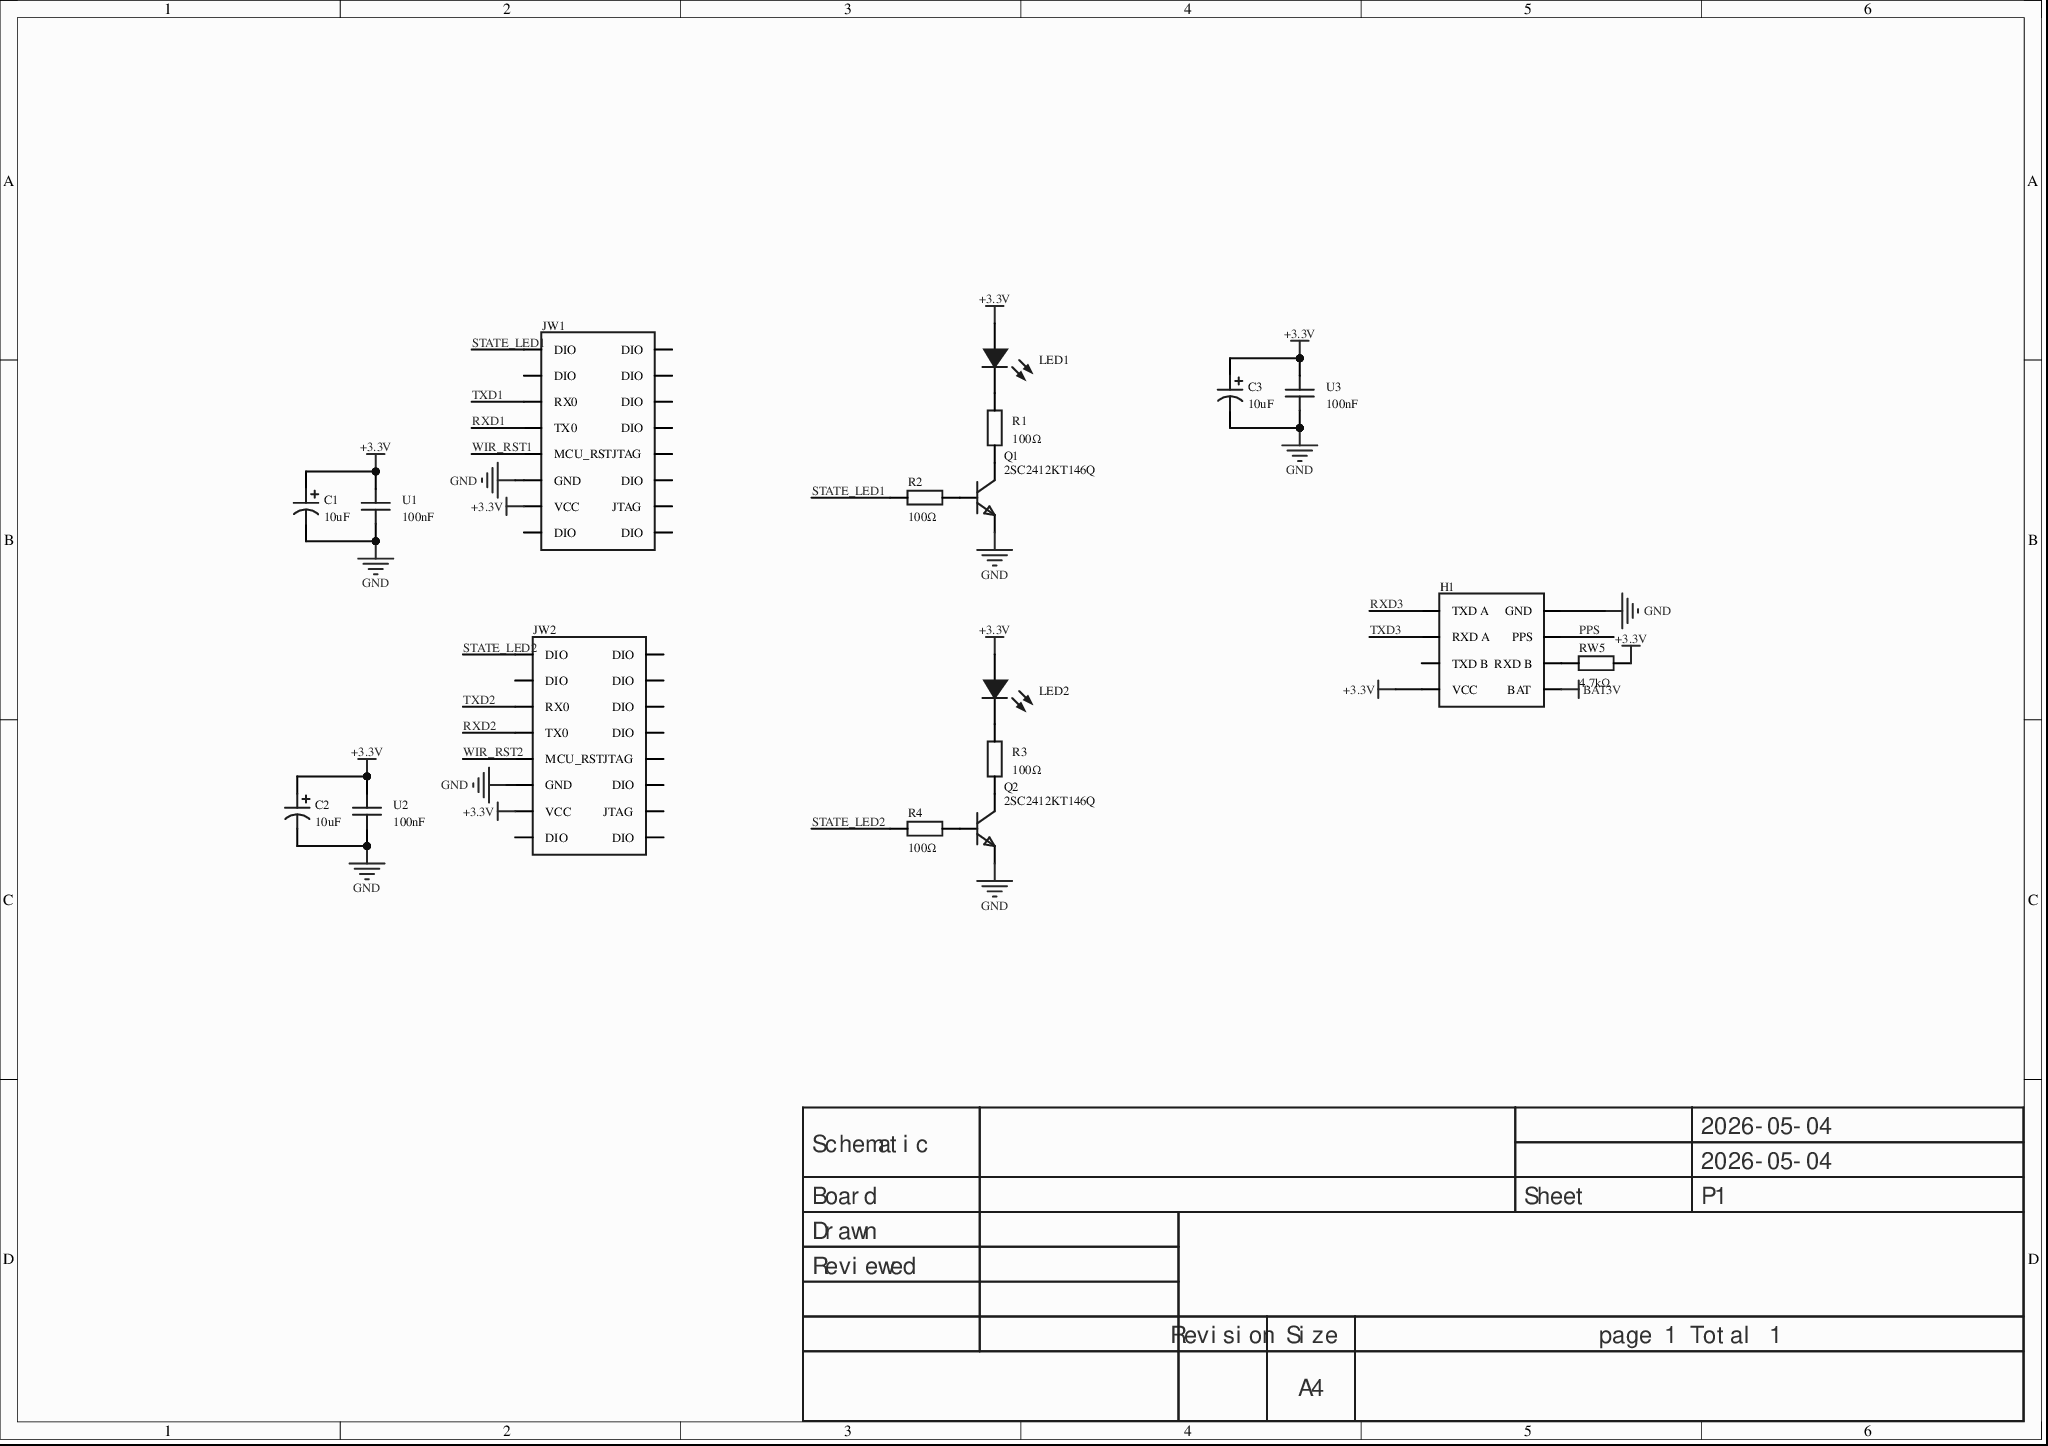
[diagram p0: MISC82880-3.schdoc]
# Altium project MISC82880-2.PrjPcb
1 sheet, 18 parts. Net scope: global (net labels, ports and power ports of the same name join across sheets).
Board file: MISC82880.pcbdoc

## Sheet MISC82880-3.schdoc
size 297 x 209 mm; Version: V1.0; @Project Name: MISC82880; @Update Date: 2026-05-04; @Create Date: 2026-05-04; @Board Name: MISC82880; @Create Time: 22:28:23; @Page Count: 1; @Page No: 1; @Schematic Name: MISC82880; @Update Time: 22:28:23; Size: A4

### Parts
C1  10uF  [CAP-TH_BD5.0-P2.00-D0.8-FD-10UF50VC110GL]
C2  10uF  [CAP-TH_BD5.0-P2.00-D0.8-FD-10UF50VC110GL]
C3  10uF  [CAP-TH_BD5.0-P2.00-D0.8-FD-10UF50VC110GL]
H1  (no value)  [HDR-TH_8P-P2.54-V-F-R2-C4-S2.54-1]
JW1  (no value)  [HDR-TH_16P-P2.54-V-F-R2-C8-S2.54-1]
JW2  (no value)  [HDR-TH_16P-P2.54-V-F-R2-C8-S2.54-1]
LED1  (no value)  [LED_TH-3mm]
LED2  (no value)  [LED_TH-3mm]
Q1  2SC2412KT146Q  [SOT-346_L2.9-W1.6-P1.90-LS2.8-TR-CW-1]
Q2  2SC2412KT146Q  [SOT-346_L2.9-W1.6-P1.90-LS2.8-TR-CW-1]
R1  100Ω  [Res_1/8W]
R2  100Ω  [Res_1/8W]
R3  100Ω  [Res_1/8W]
R4  100Ω  [Res_1/8W]
RW5  4.7kΩ  [Res_1/8W]
U1  100nF  [CAP-TH_L5.0-W2.5-P5.00-D1.0]
U2  100nF  [CAP-TH_L5.0-W2.5-P5.00-D1.0]
U3  100nF  [CAP-TH_L5.0-W2.5-P5.00-D1.0]

### Nets
+3.3V: C1.1 C2.1 C3.1 H1.7(VCC) JW1.13(VCC) JW2.13(VCC) LED1.1(C) LED2.1(C) RW5.2 U1.1 U2.1 U3.1
BAT3V: H1.8(BAT)
GND: C1.2 C2.2 C3.2 H1.2(GND) JW1.11(GND) JW2.11(GND) Q1.1(E) Q2.1(E) U1.2 U2.2 U3.2
PPS: H1.4(PPS)
RXD1: JW1.7(TX0)
RXD2: JW2.7(TX0)
RXD3: H1.1(TXD_A)
STATE_LED1: JW1.1(DIO) R2.2
STATE_LED2: JW2.1(DIO) R4.2
TXD1: JW1.5(RX0)
TXD2: JW2.5(RX0)
TXD3: H1.3(RXD_A)
WIR_RST1: JW1.9(MCU_RST)
WIR_RST2: JW2.9(MCU_RST)
NetH1_6: H1.6(RXD_B) RW5.1
NetLED1_2: LED1.2(A) R1.2
NetLED2_2: LED2.2(A) R3.2
NetQ1_2: Q1.2(B) R2.1
NetQ1_3: Q1.3(C) R1.1
NetQ2_2: Q2.2(B) R4.1
NetQ2_3: Q2.3(C) R3.1

Not connected (* = marked no-connect by the designer): H1 5(TXD_B); JW1 2(DIO) 3(DIO) 4(DIO) 6(DIO) 8(DIO) 10(JTAG) 12(DIO) 14(JTAG) 15(DIO) 16(DIO); JW2 2(DIO) 3(DIO) 4(DIO) 6(DIO) 8(DIO) 10(JTAG) 12(DIO) 14(JTAG) 15(DIO) 16(DIO)

### Notes on the sheet
- 2026-05-04
- Schematic
- Board
- Sheet
- P1
- Drawn
- Reviewed
- Revision
- Size
- A4
- page 1 Total 1

### Library data of the parts
C1 = 10UF50VC110GL: 容值:10uF;精度:±20%;额定电压:50V;纹波电流:120mA@100KHz;等效串联电阻(ESR):1.6Ω;; Manufacturer: Econd(米朗电子); AddInBom: yes; Tolerance: ±20%; Voltage Rating: 50V; Equivalent Series Resistance(ESR): 1.6Ω; Pin Spacing: 2mm; Lifetime: 5000hrs@105℃; Description: Capacitance:10uF;Tolerance:±20%;Rated voltage:50V;Ripple current:120mA@100KHz;Equivalent series resistance(ESR):1.6Ω;; Symbol: 10UF50VC110GL; Device: 10UF50VC110GL; LCSC Part Name: 10uF ±20% 50V; SupplierPart: C46867109; ManufacturerPart: 10UF50VC110GL; Supplier Footprint: 插件,D5xL11mm; JLCPCB Part Class: Extended Part; Datasheet: https://item.szlcsc.com/datasheet/10UF50VC110GL/49031974.html; Supplier: LCSC; ConvertToPcb: yes; FootprintName: CAP-TH_BD5.0-P2.00-D0.8-FD-10UF50VC110GL; Value: 10uF; Ripple Current: 120mA@100KHz; Diameter: 5mm; Height - Seated (Max): 11mm; Operating Temperature: -40℃~+105℃
C2 C3 = 10UF50VC110GL: 容值:10uF;精度:±20%;额定电压:50V;纹波电流:120mA@100KHz;等效串联电阻(ESR):1.6Ω;; Manufacturer: Econd(米朗电子); AddInBom: yes; Tolerance: ±20%; Voltage Rating: 50V; Equivalent Series Resistance(ESR): 1.6Ω; Pin Spacing: 2mm; Lifetime: 5000hrs@105℃; Symbol: 10UF50VC110GL; Device: 10UF50VC110GL; LCSC Part Name: 10uF ±20% 50V; SupplierPart: C46867109; ManufacturerPart: 10UF50VC110GL; Supplier Footprint: 插件,D5xL11mm; JLCPCB Part Class: Extended Part; Datasheet: https://item.szlcsc.com/datasheet/10UF50VC110GL/49031974.html; Supplier: LCSC; ConvertToPcb: yes; FootprintName: CAP-TH_BD5.0-P2.00-D0.8-FD-10UF50VC110GL; Value: 10uF; Ripple Current: 120mA@100KHz; Diameter: 5mm; Height - Seated (Max): 11mm; Operating Temperature: -40℃~+105℃
H1 = HDR-F_2.54_2x4: Symbol: HDR-F-2.54_2x4_1; ConvertToPcb: yes; ModelId: 64729f32a5874cf59655d275a66f10500819f05c4eef4c71ace90d822a990e87; ModelName: HDR2.54-F-LI-2X4P; ModelTransform: 399.999,200,0,0,0,0,0,0,-118.11; Device: HDR-F_2.54_2x4; AddInBom: yes; SupplierPart: C92271; Supplier Footprint: 插件; FootprintName: HDR-TH_8P-P2.54-V-F-R2-C4-S2.54-1
JW1 = HDR-F_2.54_2x8: Symbol: HDR-F-2.54_2x8_1; ConvertToPcb: yes; ModelId: f6b5f7d40ec74b809fbaeebc5002f6e00819f05c4eef4c71ace90d822a990e87; ModelName: HDR2.54-F-LI-2X8P; ModelTransform: 799.99844,200,0,0,0,0,0,0,-118.11; Device: HDR-F_2.54_2x8; AddInBom: yes; SupplierPart: C30734; Supplier Footprint: 插件; FootprintName: HDR-TH_16P-P2.54-V-F-R2-C8-S2.54-1
JW2 = HDR-F_2.54_2x8: Symbol: HDR-F-2.54_2x8_1; 3D Model: f6b5f7d40ec74b809fbaeebc5002f6e00819f05c4eef4c71ace90d822a990e87; 3D Model Transform: 799.99844,200,0,0,0,0,0,0,-118.11; ConvertToPcb: yes; ModelName: HDR2.54-F-LI-2X8P; Device: HDR-F_2.54_2x8; Supplier Part: C30734; Supplier Footprint: 插件; AddInBom: yes; FootprintName: HDR-TH_16P-P2.54-V-F-R2-C8-S2.54-1
LED1 LED2 = LED_TH-B_3mm: ConvertToPcb: yes; ModelId: ff771fff7070432ca3f353cf0f67af4c0819f05c4eef4c71ace90d822a990e87; ModelName: LED-TH_BD3.8-P2.54-FD_BLUE; ModelTransform: 134.36,149.37,405.47,0,0,0,-11.81,0,-196.85; Symbol: LED_TH-B; Device: LED_TH-B_3mm; AddInBom: yes; Supplier Footprint: 插件; FootprintName: LED_TH-3mm
Q1 = 2SC2412KT146Q: 晶体管类型:NPN;集电极电流(Ic):150mA;集射极击穿电压(Vceo):50V;耗散功率(Pd):200mW;直流电流增益(hFE):120@1mA,6V;; Manufacturer: ROHM(罗姆); AddInBom: yes; ModelId: a4a06993f12d4e549f90dd43379ebd720819f05c4eef4c71ace90d822a990e87; ModelTransform: 110.236,110.49517,0,0,0,0,0,0,0; type: NPN; Current - Collector(Ic): 150mA; Collector - Emitter Voltage VCEO: 50V; Pd - Power Dissipation: 200mW; Transition frequency(fT): 180MHz; Current - Collector Cutoff: 100nA; Vce Saturation(VCE(sat)): 400mV; Description: Transistor type:NPN;Collector current(Ic):150mA;Collector-emitter breakdown voltage(Vceo):50V;Power dissipation(Pd):200mW;DC current gain(hFE):120@1mA,6V;; Symbol: 2SC2412KT146Q; Device: 2SC2412KT146Q; LCSC Part Name: hfe=120~270 NPN 电流:150mA 电压:50V; SupplierPart: C79979; ManufacturerPart: 2SC2412KT146Q; Supplier Footprint: SOT-346; JLCPCB Part Class: Extended Part; Datasheet: https://item.szlcsc.com/datasheet/2SC2412KT146Q/81124.html; Supplier: LCSC; ConvertToPcb: yes; FootprintName: SOT-346_L2.9-W1.6-P1.90-LS2.8-TR-CW-1; ModelName: SOT-346_L2.9-W1.6-P1.90-LS2.8-TR-CW-1; DC Current Gain: 120@1mA,6V; Operating Temperature: -55℃~+150℃
Q2 = 2SC2412KT146Q: 晶体管类型:NPN;集电极电流(Ic):150mA;集射极击穿电压(Vceo):50V;耗散功率(Pd):200mW;直流电流增益(hFE):120@1mA,6V;; Manufacturer: ROHM(罗姆); AddInBom: yes; ModelId: a4a06993f12d4e549f90dd43379ebd720819f05c4eef4c71ace90d822a990e87; ModelTransform: 110.236,110.49517,0,0,0,0,0,0,0; type: NPN; Current - Collector(Ic): 150mA; Collector - Emitter Voltage VCEO: 50V; Pd - Power Dissipation: 200mW; Transition frequency(fT): 180MHz; Current - Collector Cutoff: 100nA; Vce Saturation(VCE(sat)): 400mV; Symbol: 2SC2412KT146Q; Device: 2SC2412KT146Q; LCSC Part Name: hfe=120~270 NPN 电流:150mA 电压:50V; SupplierPart: C79979; ManufacturerPart: 2SC2412KT146Q; Supplier Footprint: SOT-346; JLCPCB Part Class: Extended Part; Datasheet: https://item.szlcsc.com/datasheet/2SC2412KT146Q/81124.html; Supplier: LCSC; ConvertToPcb: yes; FootprintName: SOT-346_L2.9-W1.6-P1.90-LS2.8-TR-CW-1; ModelName: SOT-346_L2.9-W1.6-P1.90-LS2.8-TR-CW-1; DC Current Gain: 120@1mA,6V; Operating Temperature: -55℃~+150℃
R1-R4 RW5 = Res_AXIAL-1/8W: Symbol: Resistor; ConvertToPcb: yes; ModelId: b2b5ae7ae4c642178fe0039925c86a3f0819f05c4eef4c71ace90d822a990e87; ModelName: RES-TH_BD1.8-L3.2-P7.20-D0.4; ModelTransform: 282.86,66.88,253.09,0,0,0,0,0,-191; Device: Res_AXIAL-1/8W; AddInBom: yes; Supplier Footprint: 轴向引线; FootprintName: Res_1/8W
  R1-R4: Value: 100Ω
  RW5: Value: 4.7kΩ
U1-U3 = 100nF: Symbol: 100NF_C9900015256; AddInBom: yes; ModelId: 08e3d7481fc7486bb1b263873f51e1e10819f05c4eef4c71ace90d822a990e87; ModelName: CAP-TH_BD5.0-W2.5-P5.08; ModelTransform: 224.652,98.425,0,0,0,0,-0.005,0,-137.795; Device: 100nF; LCSC Part Name: 100nF; SupplierPart: C9900015256; ManufacturerPart: 100nF; Supplier Footprint: CAP-TH_L5.0-W2.5-P5.00-D1.0; JLCPCB Part Class: Extended Part; Supplier: LCSC; ConvertToPcb: yes; FootprintName: CAP-TH_L5.0-W2.5-P5.00-D1.0